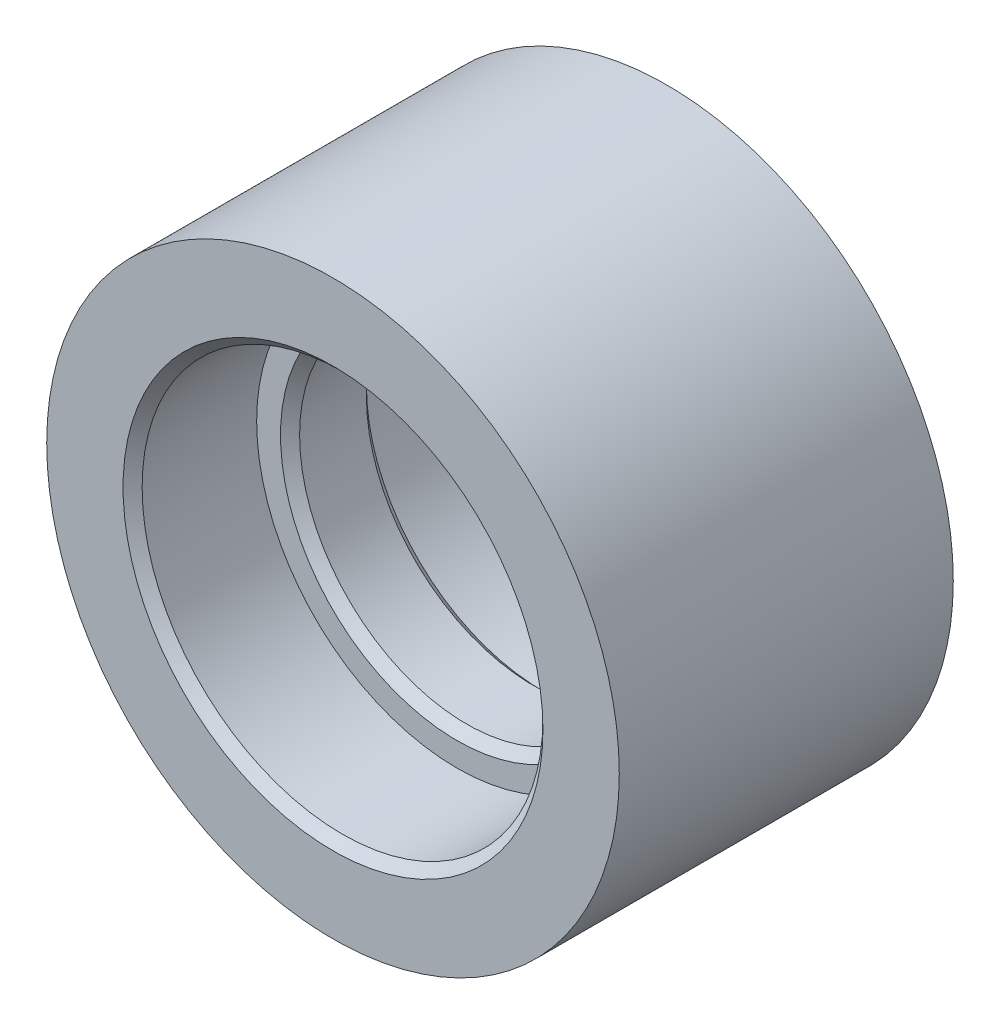
SolidWorks part; units mm, degrees
ref_plane "前视基准面" through (0, 0, 0) normal (0, 0, 1) x (1, 0, 0)
ref_plane "上视基准面" through (0, 0, 0) normal (0, 1, 0) x (1, 0, 0)
ref_plane "右视基准面" through (0, 0, 0) normal (1, 0, 0) x (0, 0, -1)
sketch "草图1" plane through (0, 0, 0) normal (0, 0, 1) x (1, 0, 0)
  circle A0 centre (0, 0) radius 30
  circle A1 centre (0, 0) radius 17.5
  dimension "D1" = 60
  dimension "D2" = 35
extrude "凸台-拉伸1" add sketch "草图1" along normal mid plane 35
sketch "草图2" plane through (0, 0, 17.5) normal (0, 0, 1) x (1, 0, 0)
  circle A0 centre (0, 0) radius 21
  dimension "D1" = 42
extrude "切除-拉伸1" cut sketch "草图2" against normal blind 13
mirror "镜向1" about plane through (0, 0, 0) normal (0, 0, 1) of "切除-拉伸1"
chamfer "倒角1" distance 1 angle 45 4 edges at (17.5, 0, 4.5) (21, 0, 17.5) (21, 0, -17.5) (-17.5, 0, -4.5)
